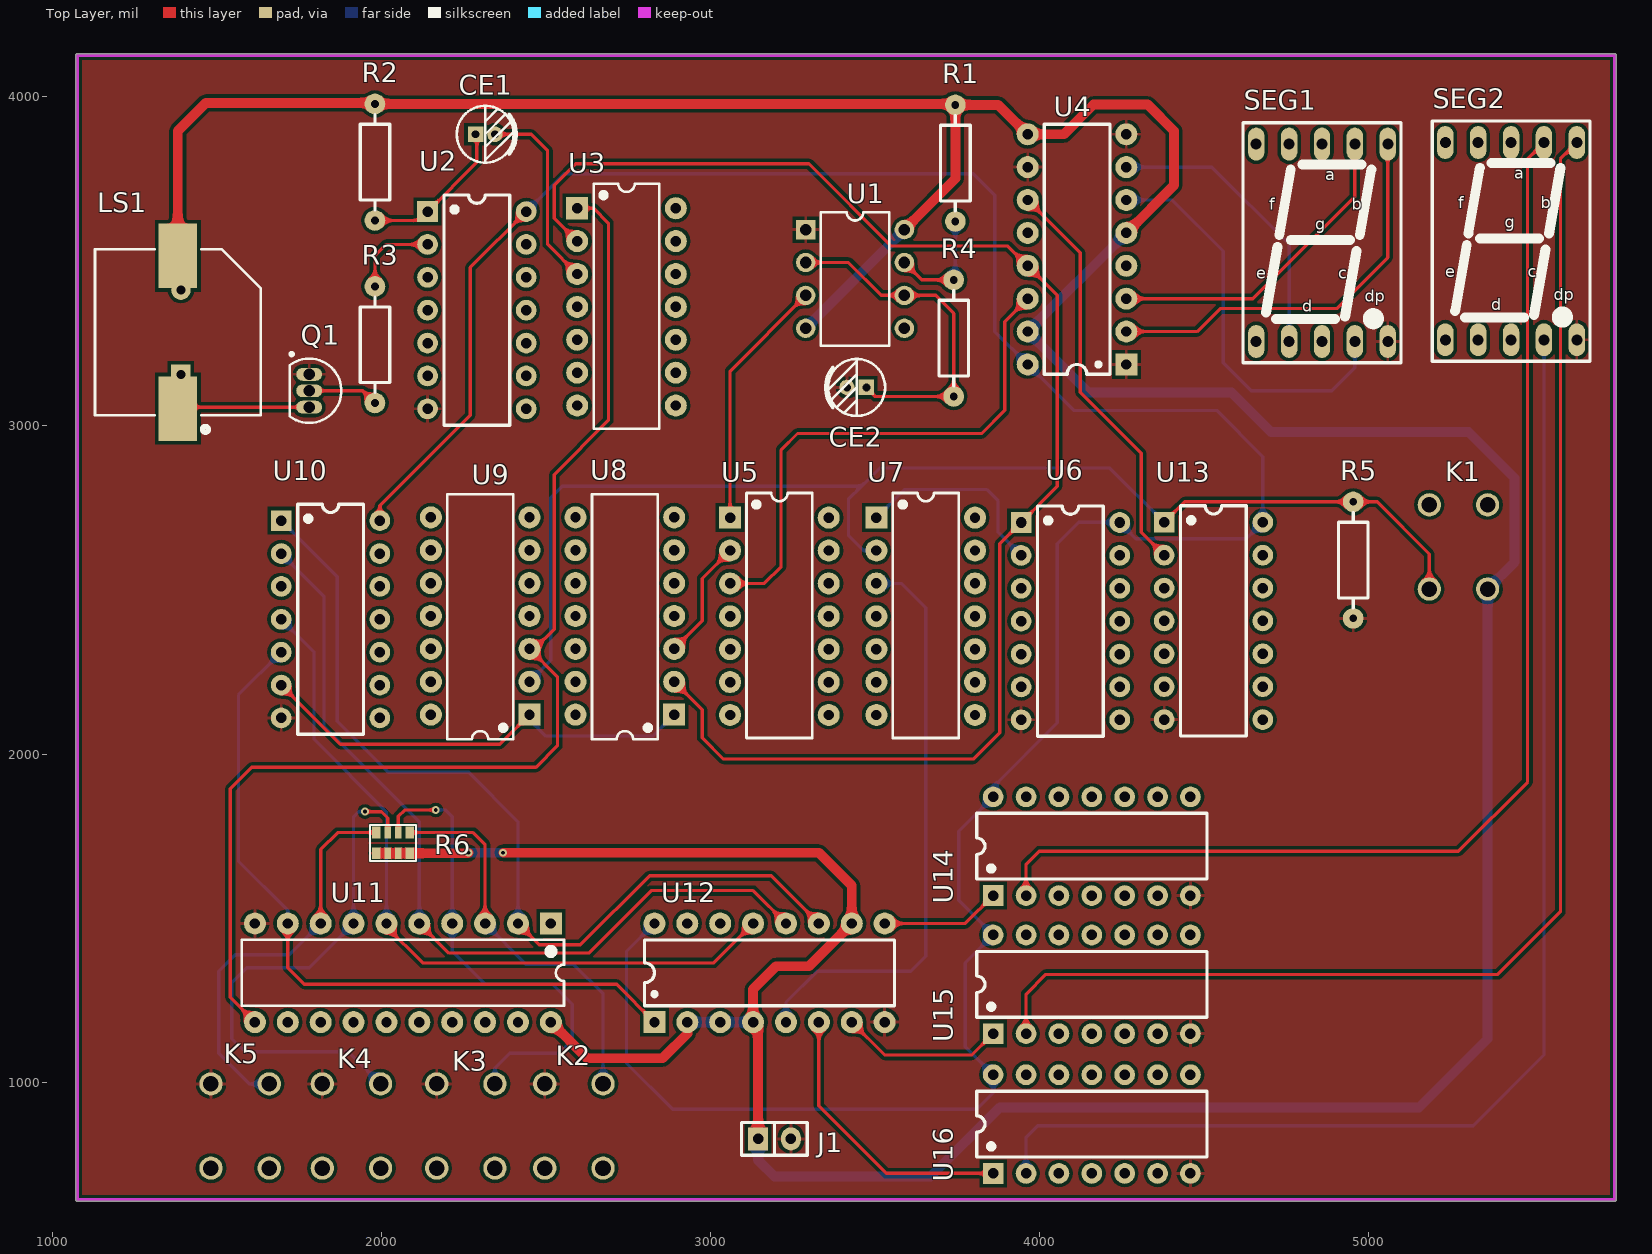
[diagram p0: Top Layer view]
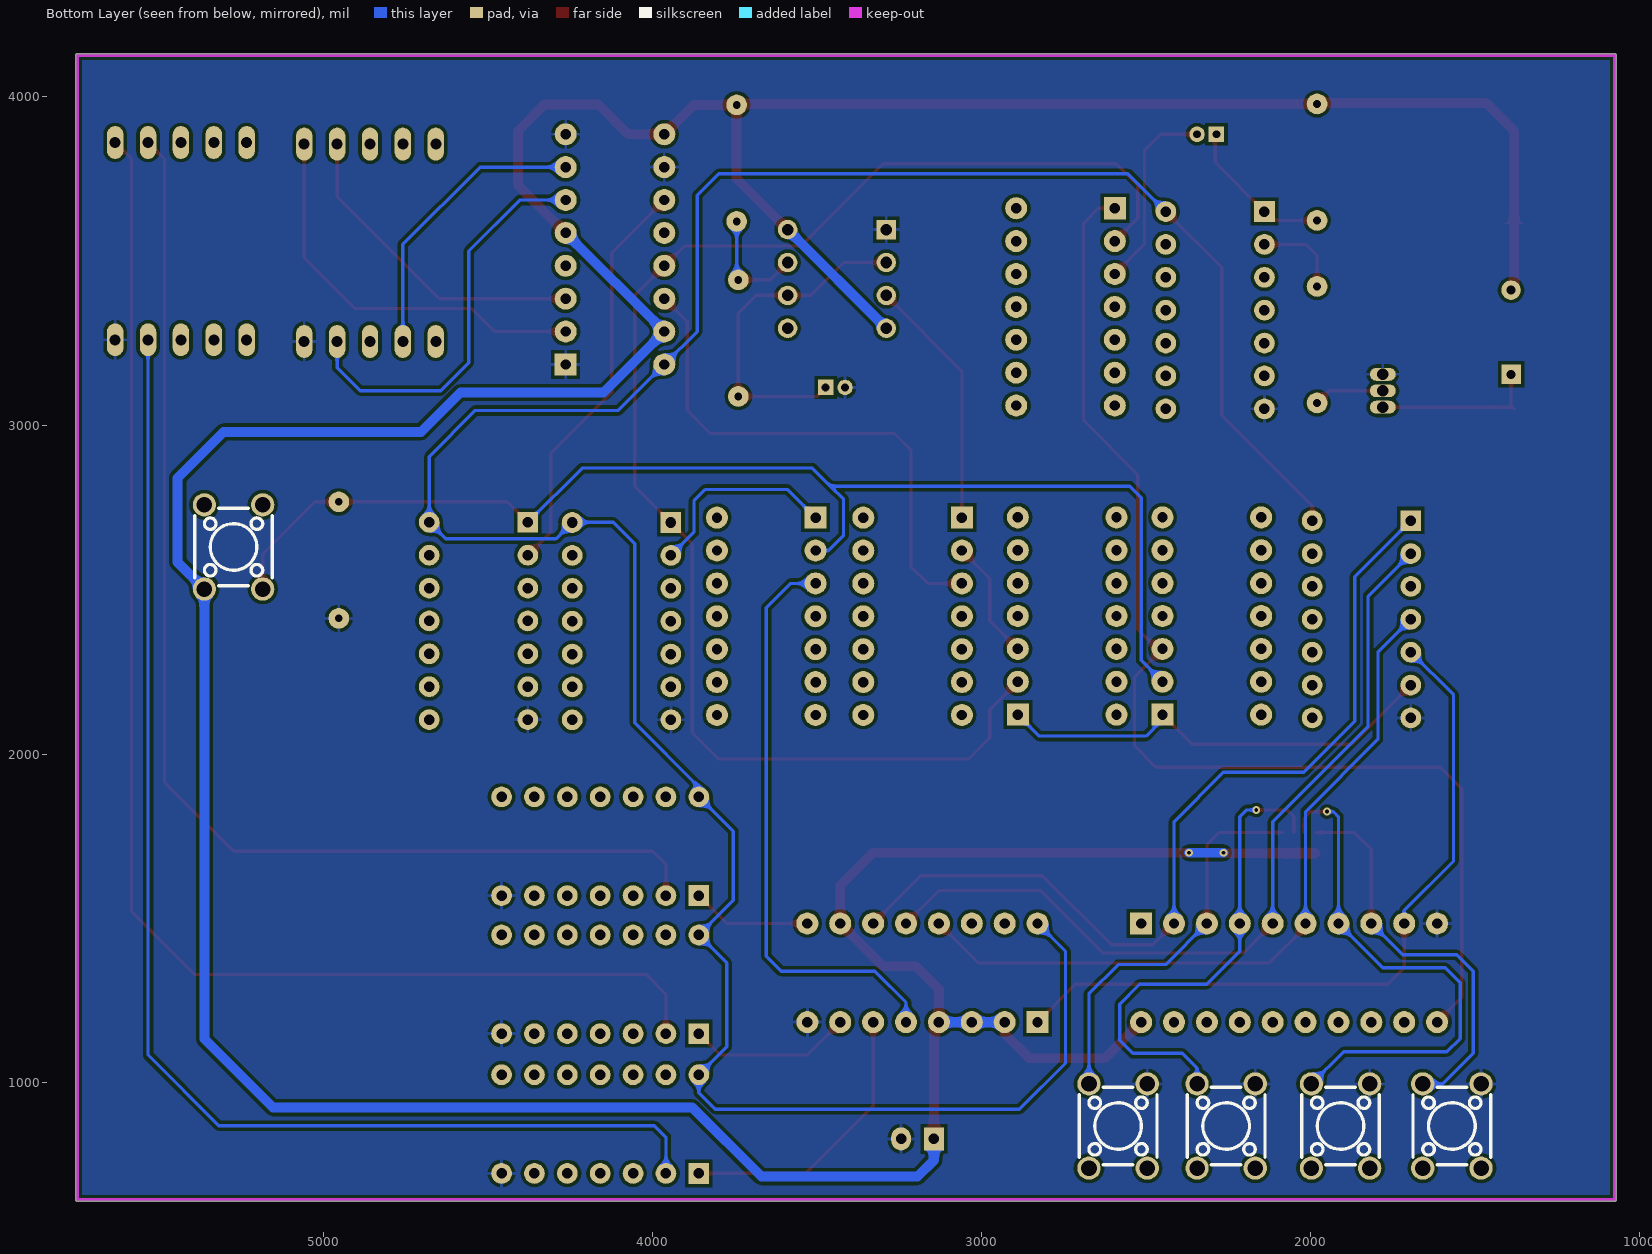
[diagram p1: Bottom Layer view, seen from below]
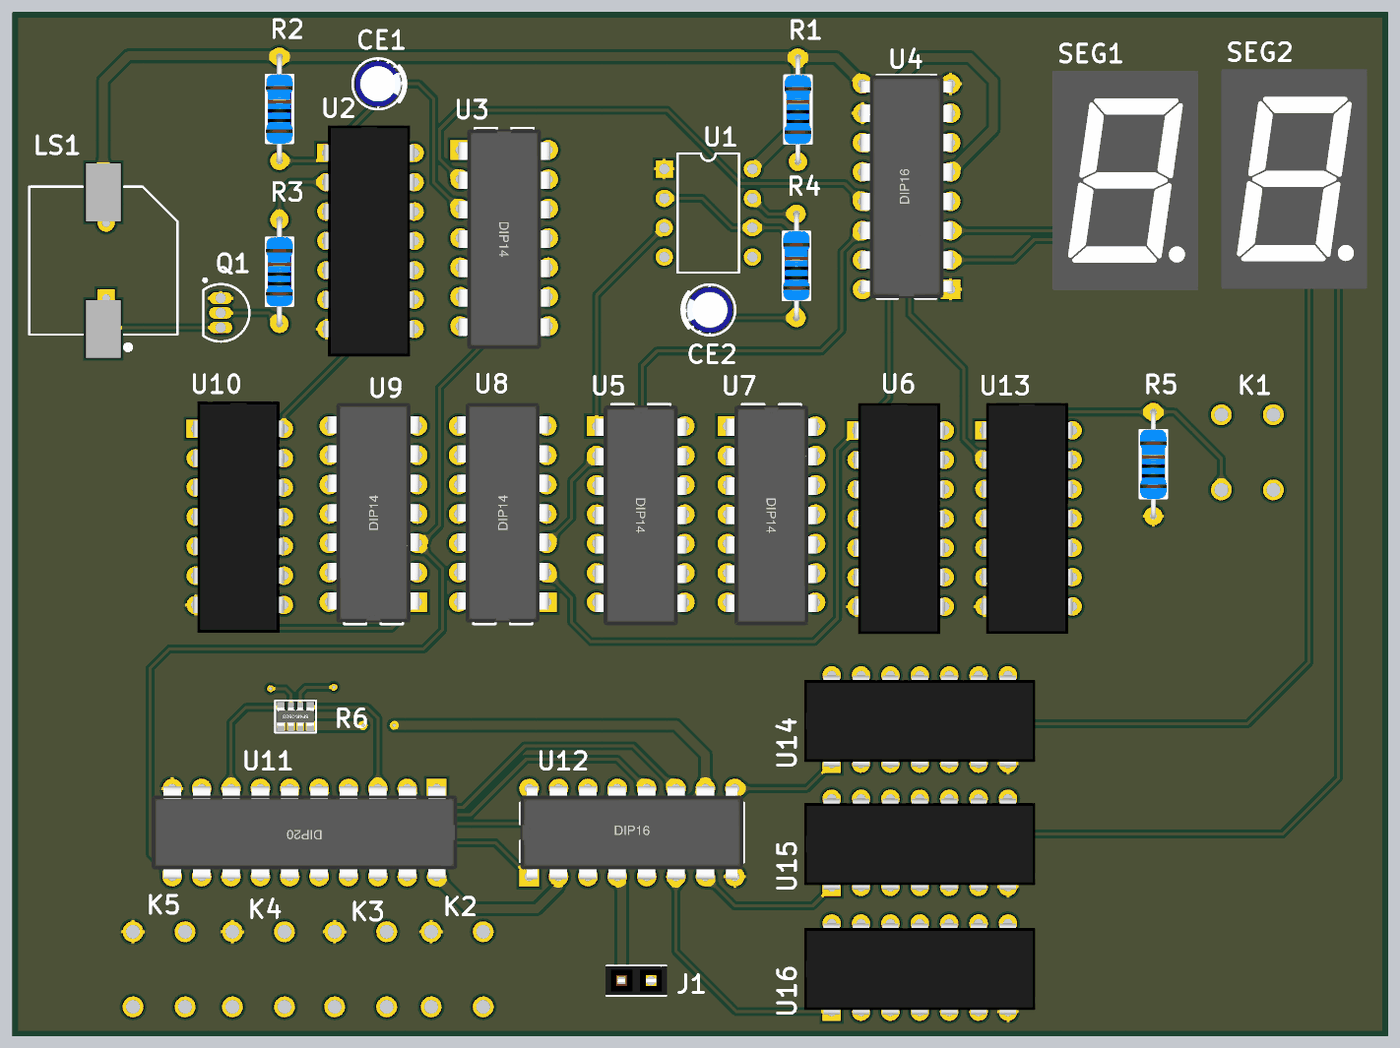
[diagram p2: 3D render of the assembled board from above, using the file's embedded part models]
# Altium PCB MISC82704.PcbDoc
Units mil, origin at the board's own origin, x right, y up, seen from the top; angles counter-clockwise.
Board outline 4685.03 x 3490.03 mil, 2 copper layers (Top Layer, Bottom Layer); 34 components, 38 nets, 299 pads, 4 vias.

## Layer stack, top to bottom (the 12.6 mil dielectric is the usual default, probably not edited)
Top Solder: solder mask 0.4, Solder Resist, Dk 3.5
Top Layer: signal copper 1.4
Dielectric 1: dielectric 12.6, FR-4, Dk 4.8
Bottom Layer: signal copper 1.4
Bottom Solder: solder mask 0.4, Solder Resist, Dk 3.5

## Board outline
1069.98,645 ccw(c1075,645) 1075,639.99 5750,639.99 ccw(c5750,645) 5755.02,645 5755.02,4125 ccw(c5750,4125) 5750,4130.02 1075,4130.02 ccw(c1075,4125) 1069.98,4125

## Design rules (kind name [scope] priority, off if disabled: settings)
Clearance [All] p1: gap=10
HoleSize [All] p1: absolutevalues=TRUE maxlimit=4444 minlimit=1 maxpercent=80.000 minpercent=20.000
MinimumSolderMaskSliver [All] p1: minsoldermaskwidth=0
PolygonConnect [All] p1: connectstyle=Relief reliefconductorwidth=10 reliefentries=4 polygonreliefangle="90 Angle" airgapwidth=10
RoutingVias [All] p1: holewidth=28 width=50 viastyle="Through Hole" minholewidth=28 minwidth=50 maxholewidth=28 maxwidth=50
SilkToSilkClearance [All] p1: silktosilkclearance=0
SilkToSolderMaskClearance [IsPad] p1: minsilkscreentomaskgap=0 clearancetoexposedcopper=TRUE
SolderMaskExpansion [All] p1: expansion=4
Width [All] p1: maxlimit=500 minlimit=10 preferedwidth=10
26 further rules are at their usual default settings.

## Components (designator, comment, footprint, x,y, rotation, side; value= is the part's Value field where it differs from the comment)
CE1 "10uF" "CAP 1.5*4*8" 2315.47,3885 r0 top
CE2 "10uF" "CAP 1.5*4*8" 3445,3115 r180 top
J1 "Female HDR1X2" Fe-HDR1X2/2.54-S 3145,830 r0 top
K1 "KEY" 四脚轻触开关 5275,2630 r270 top
K2 "KEY" 四脚轻触开关 2585,869.09 r90 top
K3 "KEY" 四脚轻触开关 2256.42,869.09 r90 top
K4 "KEY" 四脚轻触开关 1908.58,869.09 r90 top
K5 "KEY" 四脚轻触开关 1570,869.09 r90 top
LS1 "Buzzer" ABSM-1574 1380.55,3050.67 r90 top
Q1 "2N3904" TO-92A 1780,3105 r180 top
R1 "1K" "RS 1/4W" 3745,3797.17 r90 top
R2 "47K" "RS 1/4W" 1980,3800 r90 top
R3 "10K" "RS 1/4W" 1980,3245 r90 top
R4 "68K" "RS 1/4W" 3740,3265 r90 top
R5 "10K" "RS 1/4W" 4955,2590 r90 top
R6 "103" RCA-8P4R-0603 2035,1730 r180 top
SEG1 "0.56IN-1-K" 0.56IN-1P 4660,3255 r0 top
SEG2 "0.56IN-1-K" 0.56IN-1P 5235,3260 r0 top
U1 "LM555" J08A 3440,3445 r270 top
U2 "74F04N" DIP14#1 2140,3650 r0 top
U3 "74LS08" DIP14#2 2745,3360 r0 top
U4 "74LS190" DIP16 4115,3535 r180 top
U5 "74LS08" DIP14#2 3210,2419.09 r0 top
U6 "SN74F04N" DIP14#1 3945,2704.33 r0 top
U7 "74LS32" DIP14#2 3655,2419.09 r0 top
U8 "74LS08" DIP14#2 2740,2420 r180 top
U9 "74LS32" DIP14#2 2300,2420 r180 top
U10 "74LS21" DIP14#1 1695,2710 r0 top
U11 "DM74LS373N" DIP20 2065,1335 r270 top
U12 "74LS148" DIP16 3180,1335 r90 top
U13 "SN74F04N" DIP14#1 4380,2705 r0 top
U14 "SN74F04N" DIP14#1 3860,1570 r90 top
U15 "SN74F04N" DIP14#1 3860,1150 r90 top
U16 "SN74F04N" DIP14#1 3860,725 r90 top

## Footprints (in the part's own frame and the unit in brackets; to place one, negate y for a bottom-side part, rotate by r counter-clockwise, add the part's x,y. Pads: shape width x height; smd on the part's side, far side on the other; paste and mask are expansions set on the pad)
0.56IN-1P [mm]
  oval 1.27x2.54 hole 0.85: 1(0,0) 2(2.54,0) 3(5.08,0) 4(7.62,0) 5(10.16,0) 6(10.16,15.24) 7(7.62,15.24) 8(5.08,15.24) 9(2.54,15.24) 10(0,15.24)
  silkscreen extent -1.02,-1.65 11.18,16.89, body extent -1.22,-1.85 11.38,17.14, height 8
ABSM-1574 [mm] "Magnetic Transducer Buzzer"
  rect 5x3 smd: 1(0,0) 2(11.8,0)
  rect 1.5x1.5 hole 0.7: 1A(2.65,-0.24)
  round 1.5 hole 0.7: 2A(9.15,-0.24)
  silkscreen extent -1.83,-6.4 12.3,6.4
"CAP 1.5*4*8" [mm] "脚距1.5mm直径4mm高度8mm"
  rect 1.2x1.2 hole 0.6: 1(-0.75,0)
  round 1.2 hole 0.6: 2(0.75,0)
  silkscreen extent -2.2,-2.2 2.41,2.2, body extent -2,-2 2.02,2, height 8.04
DIP14#1 [mm]
  rect 1.6x1.6 hole 0.813: 1(0,0)
  round 1.6 hole 0.813: 2(0,-2.54) 3(0,-5.08) 4(0,-7.62) 5(0,-10.16) 6(0,-12.7) 7(0,-15.24) 8(7.62,-15.24) 9(7.62,-12.7) 10(7.62,-10.16) 11(7.62,-7.62) 12(7.62,-5.08) 13(7.62,-2.54) 14(7.62,0)
  silkscreen extent 1.27,-16.51 6.35,1.27, body extent -0.25,-17.62 7.62,2.38, height 5.1
DIP14#2 [mm]
  rect 1.7x1.7 hole 0.8: 1(-3.81,7.62)
  round 1.7 hole 0.8: 2(-3.81,5.08) 3(-3.81,2.54) 4(-3.81,0) 5(-3.81,-2.54) 6(-3.81,-5.08) 7(-3.81,-7.62) 8(3.81,-7.62) 9(3.81,-5.08) 10(3.81,-2.54) 11(3.81,0) 12(3.81,2.54) 13(3.81,5.08) 14(3.81,7.62)
  silkscreen extent -2.54,-9.4 2.54,9.53, body extent -3.98,-9.6 3.98,9.4, height 4.1
DIP16 [mm]
  rect 1.7x1.7 hole 0.8: 1(-3.81,8.89)
  round 1.7 hole 0.8: 2(-3.81,6.35) 3(-3.81,3.81) 4(-3.81,1.27) 5(-3.81,-1.27) 6(-3.81,-3.81) 7(-3.81,-6.35) 8(-3.81,-8.89) 9(3.81,-8.89) 10(3.81,-6.35) 11(3.81,-3.81) 12(3.81,-1.27) 13(3.81,1.27) 14(3.81,3.81) 15(3.81,6.35) 16(3.81,8.89)
  silkscreen extent -2.54,-9.65 2.54,9.65, body extent -4.02,-9.65 4.02,9.65, height 4.45
DIP20 [mm]
  rect 1.7x1.7 hole 0.8: 1(-3.81,11.43)
  round 1.7 hole 0.8: 2(-3.81,8.89) 3(-3.81,6.35) 4(-3.81,3.81) 5(-3.81,1.27) 6(-3.81,-1.27) 7(-3.81,-3.81) 8(-3.81,-6.35) 9(-3.81,-8.89) 10(-3.81,-11.43) 11(3.81,-11.43) 12(3.81,-8.89) 13(3.81,-6.35) 14(3.81,-3.81) 15(3.81,-1.27) 16(3.81,1.27) 17(3.81,3.81) 18(3.81,6.35) 19(3.81,8.89) 20(3.81,11.43)
  silkscreen extent -2.54,-12.45 2.54,12.45, body extent -4,-13.19 4,13.21, height 4.54
Fe-HDR1X2/2.54-S [mil] "Connector; Header; 2x2 Position"
  rect 60x70 hole 32: 1(0,0)
  oval 60x70 hole 32: 2(100,0)
  silkscreen extent -50,-50 150,50, body extent -55,-48 155,50, height 335
J08A [mm] "DIP; 8 Leads; Row Spacing 7.62 mm; Pitch 2.54 mm"
  rect 1.5x1.5 hole 0.9: 1(-3.81,-3.81)
  round 1.5 hole 0.9: 2(-1.27,-3.81) 3(1.27,-3.81) 4(3.81,-3.81) 5(3.81,3.81) 6(1.27,3.81) 7(-1.27,3.81) 8(-3.81,3.81)
  silkscreen extent -5.15,-2.65 5.15,2.65
RCA-8P4R-0603 [mm] "3.2mm*1.6mm*0.6mm(长*宽*厚)"
  rect 0.65x0.9 smd: 1(-1.28,-0.8) 4(1.28,-0.8) 5(1.28,0.8) 8(-1.28,0.8)
  rect 0.5x0.9 smd: 2(-0.4,-0.8) 3(0.4,-0.8) 6(0.4,0.8) 7(-0.4,0.8)
  silkscreen extent -1.78,-1.4 1.78,1.4, body extent -1.6,-0.8 1.6,0.8, height 0.6
"RS 1/4W" [mm] "直插色环电阻，脚距9mm，直径2.3mm"
  round 1.6 hole 0.6: 1(-4.5,0) 2(4.5,0)
  silkscreen extent -3.68,-1.14 3.68,1.14, body extent -4.72,-1.16 4.73,1.16, height 2.32
TO-92A [mm] "TO, Flat Index; 3 In-Line, Axial Leads; Body Dia. 4.5mm; Leads 0.51 x 0.48 mm (max)"
  oval 2x1 hole 0.9: 1(0,-1.27) 2(0,0) 3(0,1.27)
  silkscreen extent -2.48,-2.95 1.5,2.48, body extent -2.48,-2.5 1.5,2.5, height 6.86
四脚轻触开关 [mm]
  round 1.8 hole 1.2 paste+0 mask+0.102: 1(3.25,2.25) 2(-3.25,2.25) 3(3.25,-2.25) 4(-3.25,-2.25)

## Part data
CE1 CE2: library part CE, "Through-hole electrolytic capacitor"
LS1: "Magnetic Transducer Buzzer"
Q1: "NPN General Purpose Amplifier"
R1 R2 R3 R4 R5: library part R-S, "Color-band resistor"
R6: library part R-8P4R, "SMD resistor network"
SEG1 SEG2: "1-digit 0.56-inch common-cathode display"
U1: library part LM555J, "Timer"
U2: library part 74F04PC, "Hex Inverter"
U3 U5 U8: "Quad 2-input AND gate"
U4: "Synchronous 4-Bit Up/Down Decade Counter with Down/Up Mode Control"
U6 U13 U14 U15 U16: "Hex Inverter"
U7 U9: "Quad 2-input OR gate"
U10: "Dual 4-Input Positive-AND Gate"
U11: "Tri-State Octal D-Type Transparent Latch and Edge-Triggered Flip-Flop"
U12: "8-Line to 3-Line Priority Encoder"

## Via types
v1: diameter 24, hole 12, Top Layer to Bottom Layer, 4 vias

## Nets (pads, with @x,y where several pads share a name; then routed paths per layer and width w, separated by ;. In a path a pad name is that pad's centre, name@x,y a point inside that pad or via, vN(x,y) a via of type N, cw(c..) or ccw(c..) an arc to the next point about the centre after c; other vN are vias at no path point)
+5V: J1.1 K1.1 LS1.2 LS1.2A R1.2 R2.2 R6.5 R6.6 R6.7 R6.8 U1.4 U1.8 U4.5 U4.9 U4.15 U11.20 U12.2 U12.3 U12.4 U12.10 | length 14380.6
  Top Layer w30: LS1.2A 1380.55,3420.35 LS1.2 1380.55,3895.55 1465.55,3980.55 1976.61,3980.55 R2.2 3742.17,3977.17 R1.2 ; R6.5 R6.6 R6.7 R6.8 2263.5,1698.5 v1(2265,1700) ; v1(2370,1700) 3330,1700 3430,1600 U12.10 3300,1355 3200,1355 3130,1285 U12.4 3145,1170 J1.1 ; U11.20 2625,1075 2855,1075 2930,1150 U12.2 ; U1.8 3745,3750 R1.2 ; U4.5 4410,3730 4410,3895 4330,3975 4165,3975 4075,3885 U4.9 3875.67,3974.33 R1.2
  Bottom Layer w30: v1(2265,1700) v1(2370,1700) ; U12.2 U12.3 U12.4 ; J1.1 3145,765 3195,715 3670,715 3880,925 5155,925 5363.58,1133.58 K1.1 5445,2583.46 5445,2840 5305,2980 4705,2980 4585,3100 4150,3100 U4.15 U4.5 ; U1.4 U1.8
GND: CE2.2 J1.2 K2.1 K3.1 K4.1 K5.1 Q1.1 R5.1 SEG1.5 SEG2.5 U1.1 U2.7 U4.1 U4.8 U4.10 U6.7 U10.7 U11.10 U12.8 U13.7 U14.7 U15.7 U16.7
NetCE1_1: CE1.1 R2.1 U2.1 | length 470.1
  Top Layer w10: R2.1 2112.83,3622.83 U2.1 2290,3800 2290,3880.94 CE1.1
NetCE1_2: CE1.2 U3.3 | length 593
  Top Layer w10: CE1.2 2455,3885 2505,3835 2505,3550 U3.3
NetCE2_1: CE2.1 R4.1 U1.2 U1.6 | length 1043.1
  Top Layer w10: U1.2 3420,3495 3520,3395 U1.6 3685,3395 3740,3340 R4.1 3501.69,3087.83 CE2.1
NetK1_3: K1.3 R5.2 U7.2 U9.2 U13.1 | length 3832.5
  Top Layer w10: U13.1 4442.17,2767.17 R5.2 5027.83,2767.17 5186.42,2608.58 K1.3
  Bottom Layer w10: U9.2 2515,2285 2515,2780 2550,2815 3460,2815 ; U7.2 3465.91,2619.09 3420,2665 3420,2775 3460,2815 ; U13.1 4215,2870 3515,2870 3460,2815
NetK2_3: K2.3 R6.1 U11.3 | length 1206.1
  Top Layer w10: R6.1 2278.5,1761.5 2315,1725 U11.3
  Bottom Layer w10: U11.3 2440,1360 2585,1360 2673.58,1271.42 K2.3
NetK3_3: K3.3 R6.2 U11.4 | length 1499.2
  Top Layer w10: R6.2 2050.75,1810.75 2070,1830 v1(2165,1830)
  Bottom Layer w10: v1(2165,1830) 2195,1830 2215,1810 U11.4 2215,1400 2315,1300 2520,1300 2580,1240 2580,1130 2540,1090 2390,1090 2345,1045 K3.3
NetK4_3: K4.3 R6.3 U11.7 | length 1611.6
  Top Layer w10: v1(1950,1825) 2000,1825 2019.25,1805.75 R6.3
  Bottom Layer w10: v1(1950,1825) 1930,1825 1915,1810 U11.7 1780,1350 1590,1350 1545,1305 1545,1135 1585,1095 1899.21,1095 K4.3
NetK5_3: K5.3 R6.4 U11.8 | length 1228.1
  Top Layer w10: U11.8 1815,1710 1866.5,1761.5 R6.4
  Bottom Layer w10: K5.3 1597.95,997.05 1505,1090 1505,1340 1555,1390 1720,1390 U11.8
NetLS1_1: LS1.1 LS1.1A Q1.3 | length 503.4
  Top Layer w10: LS1.1 LS1.1@1384.88,3055 ; LS1.1A 1390,3060.12 LS1.1@1384.88,3055 ; Q1.3 LS1.1@1384.88,3055
NetQ1_2: Q1.2 R3.1 | length 215.4
  Top Layer w10: Q1.2 1942.83,3105 R3.1
NetR1_1: R1.1 R4.2 U1.7 | length 351.8
  Top Layer w10: U1.7 3642.83,3442.17 R4.2
  Bottom Layer w10: R4.2 3745,3447.17 R1.1
NetR3_2: R3.2 U2.2 | length 267.3
  Top Layer w10: R3.2 1980,3515 2015,3550 U2.2
NetSEG1_2: SEG1.2 U4.7 | length 887.3
  Bottom Layer w10: U4.7 4525,3785 4760,3550 SEG1.2
NetSEG1_4: SEG1.4 U4.6 | length 1243.4
  Bottom Layer w10: U4.6 4405,3685 4560,3530 4560,3190 4645,3105 4890,3105 4960,3175 SEG1.4
NetSEG1_6: SEG1.6 U4.2 | length 1233.2
  Top Layer w10: U4.2 4480,3285 4550,3355 4905,3355 5060,3510 SEG1.6
NetSEG1_7: SEG1.7 U4.3 | length 983.4
  Top Layer w10: U4.3 4650,3385 4960,3695 SEG1.7
NetSEG2_4: SEG2.4 U16.2 | length 3963.6
  Bottom Layer w10: U16.2 3960,835 3995,870 5320,870 5535,1085 SEG2.4
NetSEG2_6: SEG2.6 U15.2 | length 4209.3
  Top Layer w10: U15.2 3960,1270 4020,1330 5395,1330 5585,1520 5585,3810 SEG2.6
NetSEG2_7: SEG2.7 U14.2 | length 3689.3
  Top Layer w10: U14.2 3960,1665 4000,1705 5275,1705 5485,1915 5485,3810 SEG2.7
NetU1_3: U1.3 U5.1 | length 771.2
  Top Layer w10: U5.1 3060,3165 U1.3
NetU3_1: U3.1 U9.3 U11.11 | length 3637
  Top Layer w10: U11.11 1540,1260 1540,1895 1605,1960 2470,1960 2535,2025 2535,2235 U9.3 2465,2320 2525,2380 2525,2850 2690,3015 2690,3615 2645,3660 U3.1
NetU3_2: U3.2 U4.13 U6.1 U8.2 | length 4494.4
  Top Layer w10: U3.2 2525,3630 2525,3730 2590,3795 3300,3795 3550,3545 3905,3545 U4.13 4055,3395 4055,2814.33 U6.1 3880,2639.33 3880,2065 3800,1985 3040,1985 2975,2050 2975,2135 U8.2
NetU4_11: U4.11 U13.2 | length 1251.9
  Top Layer w10: U4.11 4125,3525 4125,3100 4310,2915 4310,2675 U13.2
NetU4_14: U4.14 U5.3 | length 1629.8
  Top Layer w10: U5.3 3164.09,2519.09 3215,2570 3215,2925 3265,2975 3825,2975 3895,3045 3895,3315 U4.14
NetU5_2: U5.2 U8.3 | length 369.5
  Top Layer w10: U8.3 2975,2405 2975,2534.09 U5.2
NetU6_2: U6.2 U7.1 | length 614.7
  Bottom Layer w10: U7.1 3590.91,2805 3840,2805 3875,2770 3875,2674.33 U6.2
NetU7_3: U7.3 U12.5 | length 1783.7
  Bottom Layer w10: U12.5 3230,1245 3325,1340 3610,1340 3655,1385 3655,2445 3580.91,2519.09 U7.3
NetU8_1: U8.1 U9.1 U10.6 | length 1369.5
  Top Layer w10: U10.6 1875,2030 2360,2030 U9.1
  Bottom Layer w10: U9.1 2450,2105 2500,2055 2825,2055 U8.1
NetU10_1: U10.1 U11.2 U12.11 | length 2755.7
  Top Layer w10: U11.2 2480,1420 2605,1420 2815,1630 3185,1630 U12.11
  Bottom Layer w10: U10.1 1865,2540 1865,2100 2020,1945 2265,1945 2415,1795 U11.2
NetU10_2: U10.2 U11.5 U12.12 | length 2571.4
  Top Layer w10: U11.5 2205,1395 2630,1395 2820,1585 3130,1585 U12.12
  Bottom Layer w10: U10.2 1825,2480 1825,2085 2115,1795 U11.5
NetU10_4: U10.4 U11.6 U12.13 | length 2277.8
  Top Layer w10: U11.6 2015,1475 2125,1365 3010,1365 U12.13
  Bottom Layer w10: U10.4 1795,2310 1795,2045 2015,1825 U11.6
NetU10_5: U10.5 U11.9 U12.1 | length 2259.3
  Top Layer w10: U11.9 1715,1350 1765,1300 2715,1300 U12.1
  Bottom Layer w10: U10.5 1565,2180 1565,1675 1715,1525 U11.9
NetU12_6: U12.6 U16.1 | length 869.9
  Top Layer w10: U12.6 3330,930 3535,725 U16.1
NetU12_7: U12.7 U15.1 | length 498.3
  Top Layer w10: U12.7 3530,1085 3795,1085 U15.1
NetU12_9: U12.9 U14.1 | length 365.2
  Top Layer w10: U12.9 3775,1485 U14.1
VCC: U2.14 U4.16 U6.14 U10.14 U12.16 U13.14 U14.14 U15.14 U16.14 | length 8466.7
  Top Layer w10: U10.14 1995,2755 2270,3030 2270,3480 U2.14
  Bottom Layer w10: U2.14 2555,3765 3800,3765 3865,3700 3865,3285 U4.16 4105,3045 4540,3045 4680,2905 U13.14 4630,2655 4294.33,2655 U6.14 4244.33,2705 4120,2705 4055,2640 4055,2095 3860,1900 U14.14 3755,1765 3755,1555 U15.14 3775,1365 3775,1110 U16.14 3860,970 3810,920 2885,920 2745,1060 2745,1400 U12.16
pads on no net: K1.2 K1.4 K2.2 K2.4 K3.2 K3.4 K4.2 K4.4 K5.2 K5.4 SEG1.1 SEG1.3 SEG1.8 SEG1.9 SEG1.10 SEG2.1 SEG2.2 SEG2.3 SEG2.8 SEG2.9 SEG2.10 U1.5 U2.3 U2.4 U2.5 U2.6 U2.8 U2.9 U2.10 U2.11 U2.12 U2.13 U3.4 U3.5 U3.6 U3.7 U3.8 U3.9 U3.10 U3.11 U3.12 U3.13 U3.14 U4.4 U4.12 U5.4 U5.5 U5.6 U5.7 U5.8 U5.9 U5.10 U5.11 U5.12 U5.13 U5.14 U6.3 U6.4 U6.5 U6.6 U6.8 U6.9 U6.10 U6.11 U6.12 U6.13 U7.4 U7.5 U7.6 U7.7 U7.8 U7.9 U7.10 U7.11 U7.12 U7.13 U7.14 U8.4 U8.5 U8.6 U8.7 U8.8 U8.9 U8.10 U8.11 U8.12 U8.13 U8.14 U9.4 U9.5 U9.6 U9.7 U9.8 U9.9 U9.10 U9.11 U9.12 U9.13 U9.14 U10.3 U10.8 U10.9 U10.10 U10.11 U10.12 U10.13 U11.1 U11.12 U11.13 U11.14 U11.15 U11.16 U11.17 U11.18 U11.19 U12.14 U12.15 U13.3 U13.4 U13.5 U13.6 U13.8 U13.9 U13.10 U13.11 U13.12 U13.13 U14.3 U14.4 U14.5 U14.6 U14.8 U14.9 U14.10 U14.11 U14.12 U14.13 U15.3 U15.4 U15.5 U15.6 U15.8 U15.9 U15.10 U15.11 U15.12 U15.13 U16.3 U16.4 U16.5 U16.6 U16.8 U16.9 U16.10 U16.11 U16.12 U16.13

## Polygon pours and split planes (outlines as drawn)
GND on Top Layer "D" (solid, remove dead copper, pour order 4): 725,4320 6130,4320 6130,470 5955,295 5750,500 645,500
GND on Bottom Layer "D" (solid, remove dead copper, pour order 6): 790,4285 6105,4285 6220,4400 6010,4190 6010,460 945,460 935,470

## Keep-outs
Keep-Out Layer:
  lines w10: 1075,4100 1075,4125 5750,4125 5750,645 1075,645 1075,4110